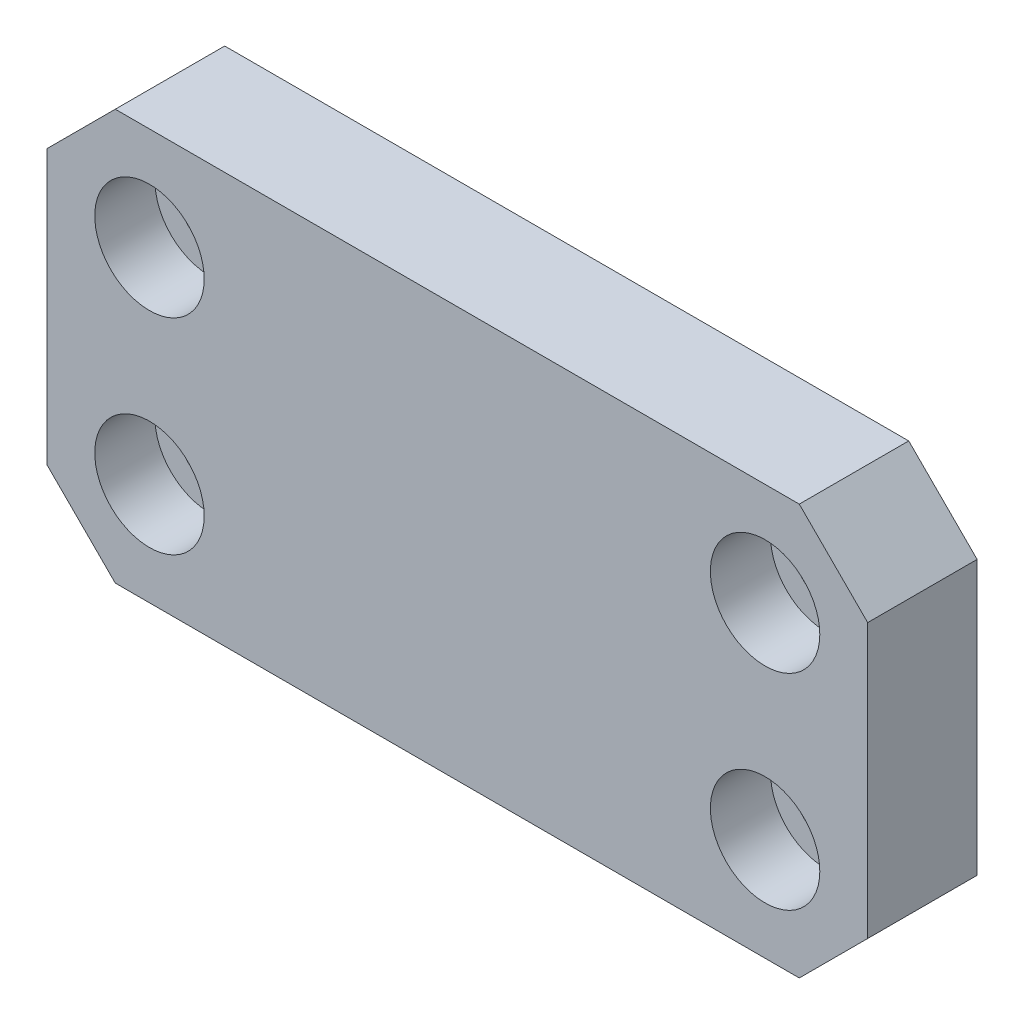
from build123d import *

# Parameters (mm, degrees)
SKETCH1_W                                           = 60
SKETCH1_H                                           = 30
BOSS_EXTRUDE1_DEPTH                                 = 8
CBORE_FOR_M4_HEX_SOCKET_HEAD_CAP_SCREW1_D           = 4.5
CBORE_FOR_M4_HEX_SOCKET_HEAD_CAP_SCREW1_CBORE_D     = 8
CBORE_FOR_M4_HEX_SOCKET_HEAD_CAP_SCREW1_CBORE_DEPTH = 4.4
CHAMFER1_SIZE                                       = 5


with BuildPart() as part:
    # Sketch1 → Boss-Extrude1 (new body)
    with BuildSketch(Plane.XY):
        Rectangle(SKETCH1_W, SKETCH1_H)
    extrude(amount=BOSS_EXTRUDE1_DEPTH)

    # CBORE for M4 Hex Socket Head Cap Screw1 (through all)
    with Locations(Plane.XY.offset(8)):
        with Locations((22.5, 7.5), (-22.5, 7.5), (-22.5, -7.5), (22.5, -7.5)):
            CounterBoreHole(CBORE_FOR_M4_HEX_SOCKET_HEAD_CAP_SCREW1_D / 2, CBORE_FOR_M4_HEX_SOCKET_HEAD_CAP_SCREW1_CBORE_D / 2, CBORE_FOR_M4_HEX_SOCKET_HEAD_CAP_SCREW1_CBORE_DEPTH)

    # Chamfer1
    chamfer1_edges = [part.edges().sort_by_distance(p)[0] for p in [
        (30, -15, 4),
        (-30, -15, 4),
        (-30, 15, 4),
        (30, 15, 4),
    ]]
    chamfer(chamfer1_edges, length=CHAMFER1_SIZE)


solid = part.part
